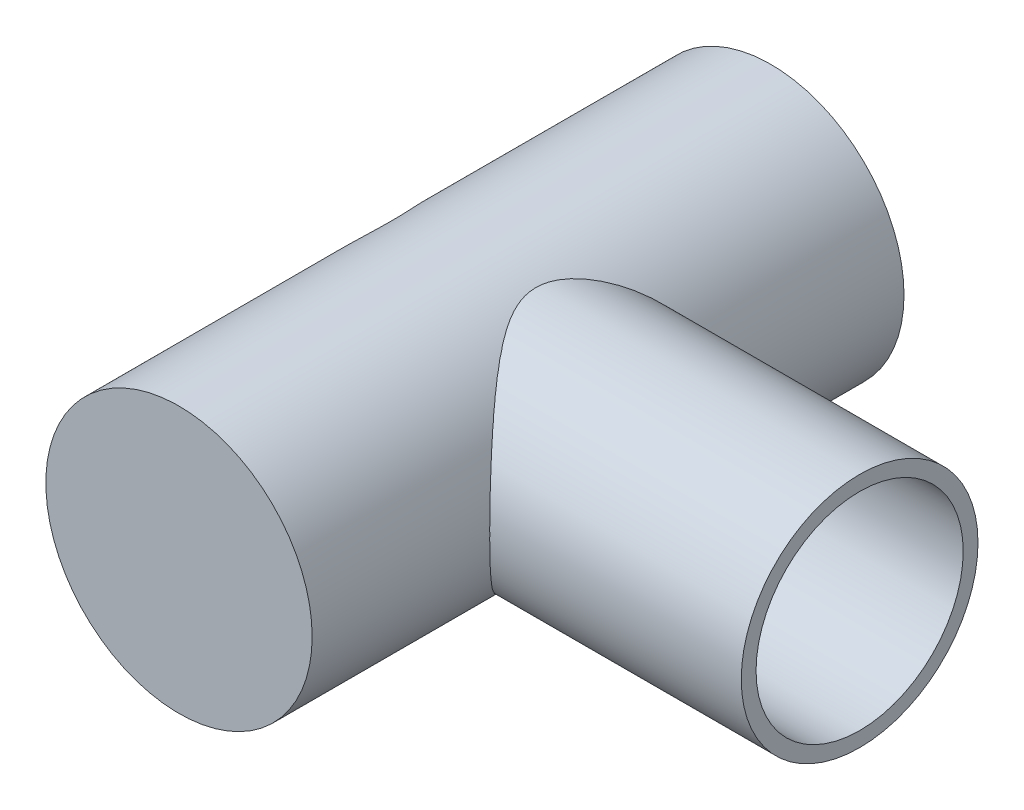
from build123d import *

# Parameters (mm, degrees)
SKETCH_1_R           = 4.5
EXTRUDE_1_DEPTH      = 20
EXTRUDE_2_REACH      = 28.954
EXTRUDE_2_END_RADIUS = 4.5
SKETCH_2_R           = 4
SKETCH_3_R           = 3.5
CUT_EXTRUDE_1_DEPTH  = 20


with BuildPart() as part:
    # 草图1 → 凸台-拉伸1 (new body)
    with BuildSketch(Plane.XY):
        Circle(SKETCH_1_R)
    extrude(amount=EXTRUDE_1_DEPTH)


with BuildPart() as body_2:
    # 凸台-拉伸2: up to this cylinder (the profile starts outside it)
    extrude_2_end = Plane(origin=(0, 0, 10), z_dir=(0, 0, -1)) * Cylinder(EXTRUDE_2_END_RADIUS, 67.908, mode=Mode.PRIVATE)
    # 草图2 → 凸台-拉伸2 (new, up to the surface)
    with BuildSketch(Plane(origin=(13, 0, 0), x_dir=(0, 0, -1), z_dir=(1, 0, 0)), mode=Mode.PRIVATE) as extrude_2_sk1:
        with Locations((-10, 0)):
            Circle(SKETCH_2_R)
    extrude_2_tool1 = extrude(extrude_2_sk1.sketch, amount=-EXTRUDE_2_REACH, mode=Mode.PRIVATE) - extrude_2_end
    add(extrude_2_tool1.solids().sort_by_distance((13, 0, 10))[0])


with BuildPart() as cut_extrude_1_tool:
    # 草图3 → 切除-拉伸1 (new body)
    with BuildSketch(Plane(origin=(13, 0, 0), x_dir=(0, 0, -1), z_dir=(1, 0, 0))):
        with Locations((-10, 0)):
            Circle(SKETCH_3_R)
    extrude(amount=-CUT_EXTRUDE_1_DEPTH)


with BuildPart() as part_1:
    add(part.part)

    # 切除-拉伸1: cut by cut_extrude_1_tool
    add(cut_extrude_1_tool.part, mode=Mode.SUBTRACT)


with BuildPart() as body_2_1:
    add(body_2.part)

    # 切除-拉伸1: cut by cut_extrude_1_tool
    add(cut_extrude_1_tool.part, mode=Mode.SUBTRACT)


solid = Compound([part_1.part, body_2_1.part])
